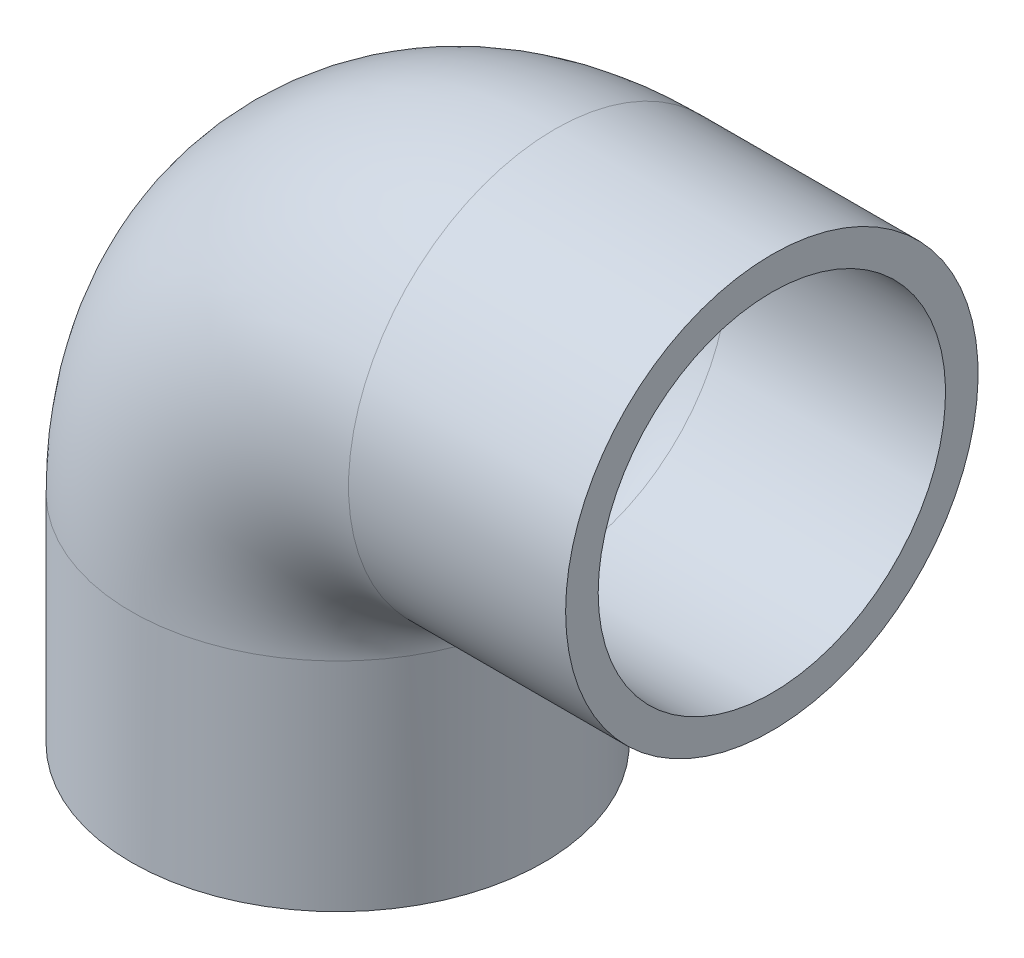
SolidWorks part; units mm, degrees
material "PP 共聚物"
ref_plane "前视基准面" through (0, 0, 0) normal (0, 0, 1) x (1, 0, 0)
ref_plane "上视基准面" through (0, 0, 0) normal (0, 1, 0) x (1, 0, 0)
ref_plane "右视基准面" through (0, 0, 0) normal (1, 0, 0) x (0, 0, -1)
sketch "草图1" plane through (0, 0, 0) normal (0, 0, 1) x (1, 0, 0)
  line L0 (0, 0) -> (0, 20)
  line L1 (20, 40) -> (40, 40)
  line L2 (40, 40) -> (0, 40) construction
  line L3 (0, 40) -> (0, 0) construction
  line L4 (16, 0) -> (19, 0) construction
  arc A0 (0, 20) -> (20, 40) centre (20, 20) cw
  dimension "D2" = 20
  dimension "a1" = 40
  dimension "dn1" = 32
  dimension "d1" = 38
sketch "草图2" plane through (0, 0, 0) normal (0, 1, 0) x (1, 0, 0)
  circle A0 centre (0, 0) radius 16
  circle A1 centre (0, 0) radius 19
sweep "扫描1" add profiles "草图2" path "草图1"
